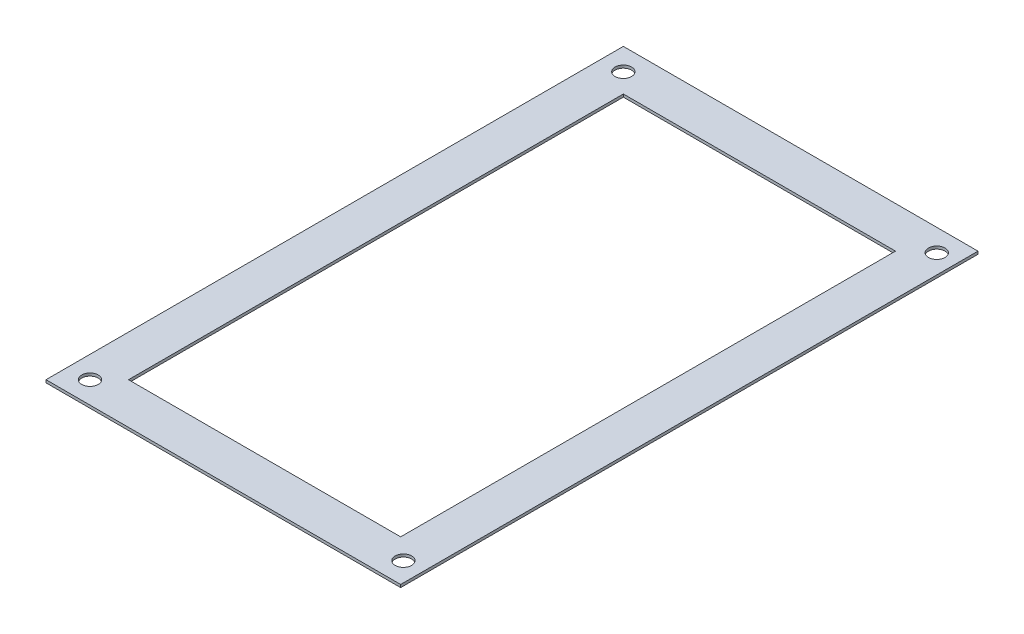
from build123d import *

# Parameters (mm, degrees)
SKETCH1_W           = 129
SKETCH1_H           = 210
SKETCH1_R           = 3
SKETCH1_W_2         = 99
SKETCH1_H_2         = 180
BOSS_EXTRUDE1_DEPTH = 1
SCALE_1_SCALE       = 1.875


with BuildPart() as part:
    # Sketch1 → Boss-Extrude1 (new body)
    with BuildSketch(Plane(origin=(0, 0, 0), x_dir=(1, 0, 0), z_dir=(0, 1, 0))):
        with Locations((23.903865936, 105)):
            Rectangle(SKETCH1_W, SKETCH1_H)
        with Locations(Location((-32.596134064, 8, 0), (0, 0, 270))):
            Circle(SKETCH1_R, mode=Mode.SUBTRACT)
        with Locations(Location((81.403865936, 8, 0), (0, 0, 270))):
            Circle(SKETCH1_R, mode=Mode.SUBTRACT)
        with Locations(Location((81.403865936, 202, 0), (0, 0, 270))):
            Circle(SKETCH1_R, mode=Mode.SUBTRACT)
        with Locations(Location((-32.596134064, 202, 0), (0, 0, 270))):
            Circle(SKETCH1_R, mode=Mode.SUBTRACT)
        with Locations((23.903865936, 105)):
            Rectangle(SKETCH1_W_2, SKETCH1_H_2, mode=Mode.SUBTRACT)
    extrude(amount=BOSS_EXTRUDE1_DEPTH)


with BuildPart() as part_1:
    # Scale 1: scaled about (23.897690412, 0.5, -105)
    add(part.part.scale(SCALE_1_SCALE).moved(Location((-20.91047911, -0.4375, 91.875))))


solid = part_1.part
